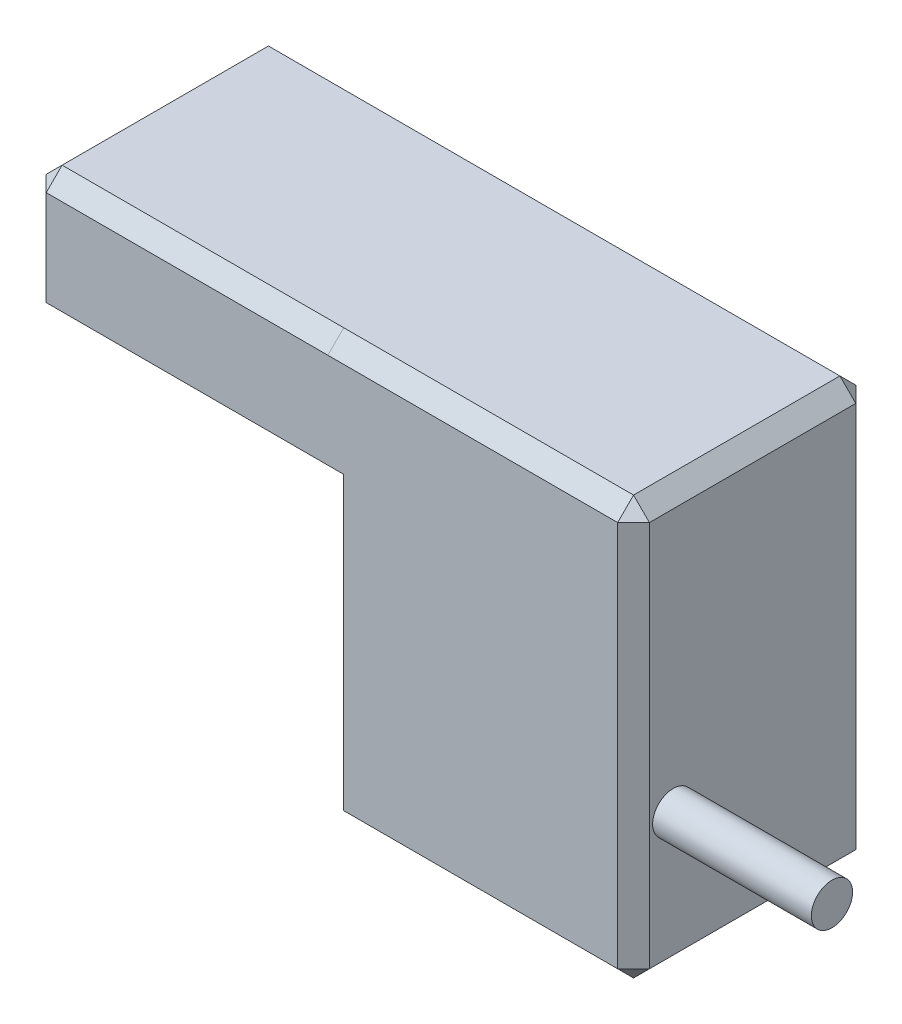
SolidWorks part; units mm, degrees
ref_plane "Front Plane" through (0, 0, 0) normal (0, 0, 1) x (1, 0, 0)
ref_plane "Top Plane" through (0, 0, 0) normal (0, 1, 0) x (1, 0, 0)
ref_plane "Right Plane" through (0, 0, 0) normal (1, 0, 0) x (0, 0, -1)
sketch "Model" plane through (0, 0, 0) normal (0, 0, 1) x (1, 0, 0)
  line L1 (-51.4146, 5.7751) -> (-51.4146, 20.7751)
  line L2 (-51.4146, 20.7751) -> (-70.6715, 20.7751)
  line L3 (-70.6715, 12.7751) -> (-70.6715, 5.7751)
  line L4 (-89.4146, 20.7751) -> (-70.6715, 20.7751)
  line L6 (-89.4146, 20.7751) -> (-89.4146, 15.7751)
  line L8 (-89.4146, 15.7751) -> (-89.4146, 12.7751)
  line L9 (-89.4146, 12.7751) -> (-70.6715, 12.7751)
  line L10 (-70.6715, 5.7751) -> (-70.6715, -5.5724)
  line L11 (-70.6715, -5.5724) -> (-51.4146, -5.5724)
  line L12 (-51.4146, -5.5724) -> (-51.4146, 5.7751)
  dimension "D1" = 15
  dimension "D2" = 18.743
  dimension "D3" = 38
  dimension "D4" = 5
  dimension "D5" = 7
extrude "Boss-Extrude1" add sketch "Model" along normal mid plane 15 contours L3 L10 L11 L12 L1 L2 L4 L6 L8 L9
sketch "Sketch3" plane through (-51.4146, 0, 0) normal (1, 0, 0) x (0, 0, -1)
  line L0 (-7.5, -5.5724) -> (-7.5, 20.7751) construction
  line L1 (7.5, -5.5724) -> (7.5, 20.7751) construction
  line L2 (-7.5, -5.5724) -> (7.5, -5.5724) construction
  circle A0 centre (-5, 3.2176) radius 1.3
  dimension "D1" = 15
  dimension "D2" = 8.79
extrude "Boss-Extrude2" add sketch "Sketch3" along normal blind 10
chamfer "Chamfer1" distance 1 angle 45 19 edges at (-89.4146, 20.7751, 0) (-51.4146, 20.7751, 0) (-61.043, 20.7751, 7.5) (-89.4146, 12.7751, 0) (-70.6715, 3.6013, -7.5) (-61.043, -5.5724, -7.5) (-80.043, 12.7751, -7.5) (-89.4146, 16.7751, -7.5) (-80.043, 20.7751, -7.5) (-61.043, 20.7751, -7.5) (-51.4146, 7.6013, -7.5) (-51.4146, 7.6013, 7.5) (-51.4146, -5.5724, 0) (-70.6715, -5.5724, 0) (-61.043, -5.5724, 7.5) (-70.6715, 3.6013, 7.5) (-80.043, 12.7751, 7.5) (-89.4146, 16.7751, 7.5) (-80.043, 20.7751, 7.5)
